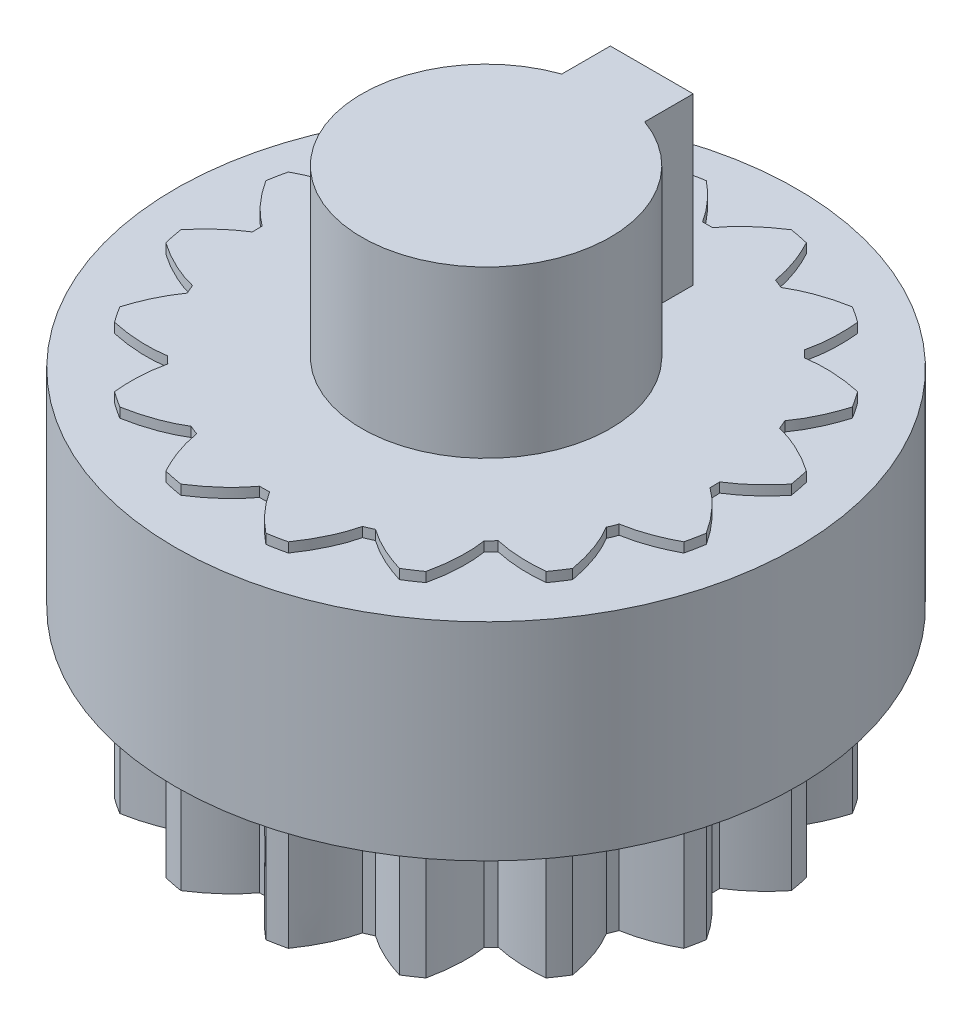
from build123d import *

# Parameters (mm, degrees)
BOSS_EXTRUDE1_DEPTH = 25
SKETCH2_R           = 15
BOSS_EXTRUDE2_DEPTH = 10
CUT_EXTRUDE1_START  = -8
CUT_EXTRUDE1_DEPTH  = 8


with BuildPart() as part:
    # Sketch1 → Boss-Extrude1 (new body)
    with BuildSketch(Plane(origin=(0, 0, 0), x_dir=(1, 0, 0), z_dir=(0, 1, 0))):
        with BuildLine():
            ThreePointArc((10.934408559, 6.749904405), (10.684384518, 7.139077494), (10.420515524, 7.518999682))
            add(Edge.make_bspline(
                [(7.734369608, 7.644942888), (7.815501047, 7.657706982), (8.159304568, 7.704570143), (8.788763458, 7.738663564), (9.465599617, 7.693246212), (10.052424346, 7.597679961), (10.374403818, 7.529145436), (10.420515524, 7.518999682)],
                knots=[0.024136697, 0.024136697, 0.024136697, 0.024136697, 0.024136697, 0.029959916, 0.048733667, 0.068727063, 0.072074856, 0.072074856, 0.072074856, 0.072074856, 0.072074856], degree=4))
            ThreePointArc((7.734369608, 7.644942888), (7.564424061, 7.813137246), (7.390821793, 7.977554652))
            add(Edge.make_bspline(
                [(7.390821793, 7.977554652), (7.395435654, 7.997349521), (7.458852977, 8.275301644), (7.549149712, 8.836196098), (7.580198449, 9.451763258), (7.554024219, 10.045742282), (7.523674581, 10.373532856), (7.518999682, 10.420515524)],
                knots=[0.028518712, 0.028518712, 0.028518712, 0.028518712, 0.028518712, 0.029959916, 0.048733667, 0.068727063, 0.072074856, 0.072074856, 0.072074856, 0.072074856, 0.072074856], degree=4))
            ThreePointArc((7.518999682, 10.420515524), (7.139077494, 10.684384518), (6.749904405, 10.934408559))
            add(Edge.make_bspline(
                [(4.220032793, 10.022821371), (4.290103862, 10.065661513), (4.589803143, 10.24052534), (5.15830034, 10.512907042), (5.800995883, 10.729960864), (6.37972286, 10.866237263), (6.703420131, 10.926135828), (6.749904405, 10.934408559)],
                knots=[0.024136697, 0.024136697, 0.024136697, 0.024136697, 0.024136697, 0.029959916, 0.048733667, 0.068727063, 0.072074856, 0.072074856, 0.072074856, 0.072074856, 0.072074856], degree=4))
            ThreePointArc((4.220032793, 10.022821371), (3.998658386, 10.11317735), (3.775350987, 10.198644514))
            add(Edge.make_bspline(
                [(3.775350987, 10.198644514), (3.77203847, 10.218698237), (3.724260764, 10.499761273), (3.593039055, 11.052515243), (3.386156994, 11.633106981), (3.134669227, 12.171855599), (2.981189795, 12.463080299), (2.958891263, 12.504697617)],
                knots=[0.028518712, 0.028518712, 0.028518712, 0.028518712, 0.028518712, 0.029959916, 0.048733667, 0.068727063, 0.072074856, 0.072074856, 0.072074856, 0.072074856, 0.072074856], degree=4))
            ThreePointArc((2.958891263, 12.504697617), (2.506910638, 12.603090853), (2.051681528, 12.685152853))
            add(Edge.make_bspline(
                [(0.06323424, 10.874816156), (0.111577253, 10.941210324), (0.321545796, 11.217453385), (0.742532756, 11.686655722), (1.253243112, 12.133136243), (1.735766401, 12.480508444), (2.011901496, 12.659721085), (2.051681528, 12.685152853)],
                knots=[0.024136697, 0.024136697, 0.024136697, 0.024136697, 0.024136697, 0.029959916, 0.048733667, 0.068727063, 0.072074856, 0.072074856, 0.072074856, 0.072074856, 0.072074856], degree=4))
            ThreePointArc((0.06323424, 10.874816156), (-0.17586678, 10.873577878), (-0.414882783, 10.8670832))
            add(Edge.make_bspline(
                [(-0.414882783, 10.8670832), (-0.425617377, 10.884342779), (-0.577316389, 11.125727429), (-0.910079227, 11.586189134), (-1.323396168, 12.04341562), (-1.761910739, 12.44491424), (-2.015154112, 12.655236743), (-2.051681528, 12.685152853)],
                knots=[0.028518712, 0.028518712, 0.028518712, 0.028518712, 0.028518712, 0.029959916, 0.048733667, 0.068727063, 0.072074856, 0.072074856, 0.072074856, 0.072074856, 0.072074856], degree=4))
            ThreePointArc((-2.051681528, 12.685152853), (-2.506910638, 12.603090853), (-2.958891263, 12.504697617))
            add(Edge.make_bspline(
                [(-4.103191153, 10.071218762), (-4.083935981, 10.151059045), (-3.995663984, 10.486625838), (-3.786278709, 11.081217009), (-3.485304562, 11.689151616), (-3.172444758, 12.194735351), (-2.985910904, 12.465978568), (-2.958891263, 12.504697617)],
                knots=[0.024136697, 0.024136697, 0.024136697, 0.024136697, 0.024136697, 0.029959916, 0.048733667, 0.068727063, 0.072074856, 0.072074856, 0.072074856, 0.072074856, 0.072074856], degree=4))
            ThreePointArc((-4.103191153, 10.071218762), (-4.323617823, 9.978574744), (-4.541954411, 9.881106979))
            add(Edge.make_bspline(
                [(-4.541954411, 9.881106979), (-4.558476837, 9.8929448), (-4.791002356, 10.057902438), (-5.274646197, 10.355970758), (-5.83147426, 10.620223405), (-6.390255767, 10.823347501), (-6.704709073, 10.920748114), (-6.749904405, 10.934408559)],
                knots=[0.028518712, 0.028518712, 0.028518712, 0.028518712, 0.028518712, 0.029959916, 0.048733667, 0.068727063, 0.072074856, 0.072074856, 0.072074856, 0.072074856, 0.072074856], degree=4))
            ThreePointArc((-6.749904405, 10.934408559), (-7.139077494, 10.684384518), (-7.518999682, 10.420515524))
            add(Edge.make_bspline(
                [(-7.644942888, 7.734369608), (-7.657706982, 7.815501047), (-7.704570143, 8.159304568), (-7.738663564, 8.788763458), (-7.693246212, 9.465599617), (-7.597679961, 10.052424346), (-7.529145436, 10.374403818), (-7.518999682, 10.420515524)],
                knots=[0.024136697, 0.024136697, 0.024136697, 0.024136697, 0.024136697, 0.029959916, 0.048733667, 0.068727063, 0.072074856, 0.072074856, 0.072074856, 0.072074856, 0.072074856], degree=4))
            ThreePointArc((-7.644942888, 7.734369608), (-7.813137246, 7.564424061), (-7.977554652, 7.390821793))
            add(Edge.make_bspline(
                [(-7.977554652, 7.390821793), (-7.997349521, 7.395435654), (-8.275301644, 7.458852977), (-8.836196098, 7.549149712), (-9.451763258, 7.580198449), (-10.045742282, 7.554024219), (-10.373532856, 7.523674581), (-10.420515524, 7.518999682)],
                knots=[0.028518712, 0.028518712, 0.028518712, 0.028518712, 0.028518712, 0.029959916, 0.048733667, 0.068727063, 0.072074856, 0.072074856, 0.072074856, 0.072074856, 0.072074856], degree=4))
            ThreePointArc((-10.420515524, 7.518999682), (-10.684384518, 7.139077494), (-10.934408559, 6.749904405))
            add(Edge.make_bspline(
                [(-10.022821371, 4.220032793), (-10.065661513, 4.290103862), (-10.24052534, 4.589803143), (-10.512907042, 5.15830034), (-10.729960864, 5.800995883), (-10.866237263, 6.37972286), (-10.926135828, 6.703420131), (-10.934408559, 6.749904405)],
                knots=[0.024136697, 0.024136697, 0.024136697, 0.024136697, 0.024136697, 0.029959916, 0.048733667, 0.068727063, 0.072074856, 0.072074856, 0.072074856, 0.072074856, 0.072074856], degree=4))
            ThreePointArc((-10.022821371, 4.220032793), (-10.11317735, 3.998658386), (-10.198644514, 3.775350987))
            add(Edge.make_bspline(
                [(-10.198644514, 3.775350987), (-10.218698237, 3.77203847), (-10.499761273, 3.724260764), (-11.052515243, 3.593039055), (-11.633106981, 3.386156994), (-12.171855599, 3.134669227), (-12.463080299, 2.981189795), (-12.504697617, 2.958891263)],
                knots=[0.028518712, 0.028518712, 0.028518712, 0.028518712, 0.028518712, 0.029959916, 0.048733667, 0.068727063, 0.072074856, 0.072074856, 0.072074856, 0.072074856, 0.072074856], degree=4))
            ThreePointArc((-12.504697617, 2.958891263), (-12.603090853, 2.506910638), (-12.685152853, 2.051681528))
            add(Edge.make_bspline(
                [(-10.874816156, 0.06323424), (-10.941210324, 0.111577253), (-11.217453385, 0.321545796), (-11.686655722, 0.742532756), (-12.133136243, 1.253243112), (-12.480508444, 1.735766401), (-12.659721085, 2.011901496), (-12.685152853, 2.051681528)],
                knots=[0.024136697, 0.024136697, 0.024136697, 0.024136697, 0.024136697, 0.029959916, 0.048733667, 0.068727063, 0.072074856, 0.072074856, 0.072074856, 0.072074856, 0.072074856], degree=4))
            ThreePointArc((-10.874816156, 0.06323424), (-10.873577878, -0.17586678), (-10.8670832, -0.414882783))
            add(Edge.make_bspline(
                [(-10.8670832, -0.414882783), (-10.884342779, -0.425617377), (-11.125727429, -0.577316389), (-11.586189134, -0.910079227), (-12.04341562, -1.323396168), (-12.44491424, -1.761910739), (-12.655236743, -2.015154112), (-12.685152853, -2.051681528)],
                knots=[0.028518712, 0.028518712, 0.028518712, 0.028518712, 0.028518712, 0.029959916, 0.048733667, 0.068727063, 0.072074856, 0.072074856, 0.072074856, 0.072074856, 0.072074856], degree=4))
            ThreePointArc((-12.685152853, -2.051681528), (-12.603090853, -2.506910638), (-12.504697617, -2.958891263))
            add(Edge.make_bspline(
                [(-10.071218762, -4.103191153), (-10.151059045, -4.083935981), (-10.486625838, -3.995663984), (-11.081217009, -3.786278709), (-11.689151616, -3.485304562), (-12.194735351, -3.172444758), (-12.465978568, -2.985910904), (-12.504697617, -2.958891263)],
                knots=[0.024136697, 0.024136697, 0.024136697, 0.024136697, 0.024136697, 0.029959916, 0.048733667, 0.068727063, 0.072074856, 0.072074856, 0.072074856, 0.072074856, 0.072074856], degree=4))
            ThreePointArc((-10.071218762, -4.103191153), (-9.978574744, -4.323617823), (-9.881106979, -4.541954411))
            add(Edge.make_bspline(
                [(-9.881106979, -4.541954411), (-9.8929448, -4.558476837), (-10.057902438, -4.791002356), (-10.355970758, -5.274646197), (-10.620223405, -5.83147426), (-10.823347501, -6.390255767), (-10.920748114, -6.704709073), (-10.934408559, -6.749904405)],
                knots=[0.028518712, 0.028518712, 0.028518712, 0.028518712, 0.028518712, 0.029959916, 0.048733667, 0.068727063, 0.072074856, 0.072074856, 0.072074856, 0.072074856, 0.072074856], degree=4))
            ThreePointArc((-10.934408559, -6.749904405), (-10.684384518, -7.139077494), (-10.420515524, -7.518999682))
            add(Edge.make_bspline(
                [(-7.734369608, -7.644942888), (-7.815501047, -7.657706982), (-8.159304568, -7.704570143), (-8.788763458, -7.738663564), (-9.465599617, -7.693246212), (-10.052424346, -7.597679961), (-10.374403818, -7.529145436), (-10.420515524, -7.518999682)],
                knots=[0.024136697, 0.024136697, 0.024136697, 0.024136697, 0.024136697, 0.029959916, 0.048733667, 0.068727063, 0.072074856, 0.072074856, 0.072074856, 0.072074856, 0.072074856], degree=4))
            ThreePointArc((-7.734369608, -7.644942888), (-7.564424061, -7.813137246), (-7.390821793, -7.977554652))
            add(Edge.make_bspline(
                [(-7.390821793, -7.977554652), (-7.395435654, -7.997349521), (-7.458852977, -8.275301644), (-7.549149712, -8.836196098), (-7.580198449, -9.451763258), (-7.554024219, -10.045742282), (-7.523674581, -10.373532856), (-7.518999682, -10.420515524)],
                knots=[0.028518712, 0.028518712, 0.028518712, 0.028518712, 0.028518712, 0.029959916, 0.048733667, 0.068727063, 0.072074856, 0.072074856, 0.072074856, 0.072074856, 0.072074856], degree=4))
            ThreePointArc((-7.518999682, -10.420515524), (-7.139077494, -10.684384518), (-6.749904405, -10.934408559))
            add(Edge.make_bspline(
                [(-4.220032793, -10.022821371), (-4.290103862, -10.065661513), (-4.589803143, -10.24052534), (-5.15830034, -10.512907042), (-5.800995883, -10.729960864), (-6.37972286, -10.866237263), (-6.703420131, -10.926135828), (-6.749904405, -10.934408559)],
                knots=[0.024136697, 0.024136697, 0.024136697, 0.024136697, 0.024136697, 0.029959916, 0.048733667, 0.068727063, 0.072074856, 0.072074856, 0.072074856, 0.072074856, 0.072074856], degree=4))
            ThreePointArc((-4.220032793, -10.022821371), (-3.998658386, -10.11317735), (-3.775350987, -10.198644514))
            add(Edge.make_bspline(
                [(-3.775350987, -10.198644514), (-3.77203847, -10.218698237), (-3.724260764, -10.499761273), (-3.593039055, -11.052515243), (-3.386156994, -11.633106981), (-3.134669227, -12.171855599), (-2.981189795, -12.463080299), (-2.958891263, -12.504697617)],
                knots=[0.028518712, 0.028518712, 0.028518712, 0.028518712, 0.028518712, 0.029959916, 0.048733667, 0.068727063, 0.072074856, 0.072074856, 0.072074856, 0.072074856, 0.072074856], degree=4))
            ThreePointArc((-2.958891263, -12.504697617), (-2.506910638, -12.603090853), (-2.051681528, -12.685152853))
            add(Edge.make_bspline(
                [(-0.06323424, -10.874816156), (-0.111577253, -10.941210324), (-0.321545796, -11.217453385), (-0.742532756, -11.686655722), (-1.253243112, -12.133136243), (-1.735766401, -12.480508444), (-2.011901496, -12.659721085), (-2.051681528, -12.685152853)],
                knots=[0.024136697, 0.024136697, 0.024136697, 0.024136697, 0.024136697, 0.029959916, 0.048733667, 0.068727063, 0.072074856, 0.072074856, 0.072074856, 0.072074856, 0.072074856], degree=4))
            ThreePointArc((-0.06323424, -10.874816156), (0.17586678, -10.873577878), (0.414882783, -10.8670832))
            add(Edge.make_bspline(
                [(0.414882783, -10.8670832), (0.425617377, -10.884342779), (0.577316389, -11.125727429), (0.910079227, -11.586189134), (1.323396168, -12.04341562), (1.761910739, -12.44491424), (2.015154112, -12.655236743), (2.051681528, -12.685152853)],
                knots=[0.028518712, 0.028518712, 0.028518712, 0.028518712, 0.028518712, 0.029959916, 0.048733667, 0.068727063, 0.072074856, 0.072074856, 0.072074856, 0.072074856, 0.072074856], degree=4))
            ThreePointArc((2.051681528, -12.685152853), (2.506910638, -12.603090853), (2.958891263, -12.504697617))
            add(Edge.make_bspline(
                [(4.103191153, -10.071218762), (4.083935981, -10.151059045), (3.995663984, -10.486625838), (3.786278709, -11.081217009), (3.485304562, -11.689151616), (3.172444758, -12.194735351), (2.985910904, -12.465978568), (2.958891263, -12.504697617)],
                knots=[0.024136697, 0.024136697, 0.024136697, 0.024136697, 0.024136697, 0.029959916, 0.048733667, 0.068727063, 0.072074856, 0.072074856, 0.072074856, 0.072074856, 0.072074856], degree=4))
            ThreePointArc((4.103191153, -10.071218762), (4.323617823, -9.978574744), (4.541954411, -9.881106979))
            add(Edge.make_bspline(
                [(4.541954411, -9.881106979), (4.558476837, -9.8929448), (4.791002356, -10.057902438), (5.274646197, -10.355970758), (5.83147426, -10.620223405), (6.390255767, -10.823347501), (6.704709073, -10.920748114), (6.749904405, -10.934408559)],
                knots=[0.028518712, 0.028518712, 0.028518712, 0.028518712, 0.028518712, 0.029959916, 0.048733667, 0.068727063, 0.072074856, 0.072074856, 0.072074856, 0.072074856, 0.072074856], degree=4))
            ThreePointArc((6.749904405, -10.934408559), (7.139077494, -10.684384518), (7.518999682, -10.420515524))
            add(Edge.make_bspline(
                [(7.644942888, -7.734369608), (7.657706982, -7.815501047), (7.704570143, -8.159304568), (7.738663564, -8.788763458), (7.693246212, -9.465599617), (7.597679961, -10.052424346), (7.529145436, -10.374403818), (7.518999682, -10.420515524)],
                knots=[0.024136697, 0.024136697, 0.024136697, 0.024136697, 0.024136697, 0.029959916, 0.048733667, 0.068727063, 0.072074856, 0.072074856, 0.072074856, 0.072074856, 0.072074856], degree=4))
            ThreePointArc((7.644942888, -7.734369608), (7.813137246, -7.564424061), (7.977554652, -7.390821793))
            add(Edge.make_bspline(
                [(7.977554652, -7.390821793), (7.997349521, -7.395435654), (8.275301644, -7.458852977), (8.836196098, -7.549149712), (9.451763258, -7.580198449), (10.045742282, -7.554024219), (10.373532856, -7.523674581), (10.420515524, -7.518999682)],
                knots=[0.028518712, 0.028518712, 0.028518712, 0.028518712, 0.028518712, 0.029959916, 0.048733667, 0.068727063, 0.072074856, 0.072074856, 0.072074856, 0.072074856, 0.072074856], degree=4))
            ThreePointArc((10.420515524, -7.518999682), (10.684384518, -7.139077494), (10.934408559, -6.749904405))
            add(Edge.make_bspline(
                [(10.022821371, -4.220032793), (10.065661513, -4.290103862), (10.24052534, -4.589803143), (10.512907042, -5.15830034), (10.729960864, -5.800995883), (10.866237263, -6.37972286), (10.926135828, -6.703420131), (10.934408559, -6.749904405)],
                knots=[0.024136697, 0.024136697, 0.024136697, 0.024136697, 0.024136697, 0.029959916, 0.048733667, 0.068727063, 0.072074856, 0.072074856, 0.072074856, 0.072074856, 0.072074856], degree=4))
            ThreePointArc((10.022821371, -4.220032793), (10.11317735, -3.998658386), (10.198644514, -3.775350987))
            add(Edge.make_bspline(
                [(10.198644514, -3.775350987), (10.218698237, -3.77203847), (10.499761273, -3.724260764), (11.052515243, -3.593039055), (11.633106981, -3.386156994), (12.171855599, -3.134669227), (12.463080299, -2.981189795), (12.504697617, -2.958891263)],
                knots=[0.028518712, 0.028518712, 0.028518712, 0.028518712, 0.028518712, 0.029959916, 0.048733667, 0.068727063, 0.072074856, 0.072074856, 0.072074856, 0.072074856, 0.072074856], degree=4))
            ThreePointArc((12.504697617, -2.958891263), (12.603090853, -2.506910638), (12.685152853, -2.051681528))
            add(Edge.make_bspline(
                [(10.874816156, -0.06323424), (10.941210324, -0.111577253), (11.217453385, -0.321545796), (11.686655722, -0.742532756), (12.133136243, -1.253243112), (12.480508444, -1.735766401), (12.659721085, -2.011901496), (12.685152853, -2.051681528)],
                knots=[0.024136697, 0.024136697, 0.024136697, 0.024136697, 0.024136697, 0.029959916, 0.048733667, 0.068727063, 0.072074856, 0.072074856, 0.072074856, 0.072074856, 0.072074856], degree=4))
            ThreePointArc((10.874816156, -0.06323424), (10.8735779, 0.175865412), (10.867083304, 0.41488005))
            add(Edge.make_bspline(
                [(10.867083304, 0.41488005), (10.881563831, 0.423886532), (10.909967193, 0.441770581), (10.976624087, 0.484202292), (11.030614279, 0.520337558), (11.104594394, 0.570140428), (11.165588686, 0.613063664), (11.233528062, 0.661496019), (11.296306007, 0.707854009), (11.361321254, 0.756764897), (11.424005499, 0.805285781), (11.487262257, 0.855332478), (11.549125239, 0.905448576), (11.611116576, 0.956904432), (11.682171109, 1.017033988), (11.768675064, 1.092619353), (11.8667636, 1.180577496), (11.981028216, 1.288212398), (12.092602454, 1.396325305), (12.209848472, 1.516302043), (12.31227485, 1.623029301), (12.43305143, 1.756891779), (12.517769899, 1.851362852), (12.621696804, 1.974933325), (12.663559289, 2.025313794), (12.685153092, 2.05168005)],
                knots=[0.063770479, 0.063770479, 0.063770479, 0.063770479, 0.063770479, 0.091530707, 0.119271063, 0.147011529, 0.174751886, 0.202492214, 0.230232656, 0.257973071, 0.285713397, 0.313453819, 0.341194243, 0.368934578, 0.396674935, 0.424415392, 0.47104384, 0.526524589, 0.58200537, 0.637486135, 0.692966903, 0.748447704, 0.803928446, 0.859409239, 0.914890039, 0.914890039, 0.914890039, 0.914890039, 0.914890039], degree=4))
            ThreePointArc((12.685153092, 2.05168005), (12.603090999, 2.506909904), (12.504697617, 2.958891263))
            add(Edge.make_bspline(
                [(10.071218762, 4.103191153), (10.151059045, 4.083935981), (10.486625838, 3.995663984), (11.081217009, 3.786278709), (11.689151616, 3.485304562), (12.194735351, 3.172444758), (12.465978568, 2.985910904), (12.504697617, 2.958891263)],
                knots=[0.024136697, 0.024136697, 0.024136697, 0.024136697, 0.024136697, 0.029959916, 0.048733667, 0.068727063, 0.072074856, 0.072074856, 0.072074856, 0.072074856, 0.072074856], degree=4))
            ThreePointArc((10.071218762, 4.103191153), (9.978574744, 4.323617823), (9.881106979, 4.541954411))
            add(Edge.make_bspline(
                [(9.881106979, 4.541954411), (9.8929448, 4.558476837), (10.057902438, 4.791002356), (10.355970758, 5.274646197), (10.620223405, 5.83147426), (10.823347501, 6.390255767), (10.920748114, 6.704709073), (10.934408559, 6.749904405)],
                knots=[0.028518712, 0.028518712, 0.028518712, 0.028518712, 0.028518712, 0.029959916, 0.048733667, 0.068727063, 0.072074856, 0.072074856, 0.072074856, 0.072074856, 0.072074856], degree=4))
        make_face()
    extrude(amount=BOSS_EXTRUDE1_DEPTH)

    # Sketch2 → Boss-Extrude2 (add)
    with BuildSketch(Plane(origin=(0, 6.530075329, 0), x_dir=(1, 0, 0), z_dir=(0, 1, 0))):
        with Locations(Location((0, 0, 0), (0, 0, 270))):
            Circle(SKETCH2_R)
    extrude(amount=BOSS_EXTRUDE2_DEPTH)

    # Sketch3 → Cut-Extrude1 (cut)
    with BuildSketch(Plane(origin=(0, 25, 0), x_dir=(1, 0, 0), z_dir=(0, 1, 0)).offset(CUT_EXTRUDE1_START)):
        with BuildLine():
            ThreePointArc((10.874816156, -0.06323424), (10.8735779, 0.175865412), (10.867083304, 0.41488005))
            add(Edge.make_bspline(
                [(10.867083304, 0.41488005), (10.881563831, 0.423886532), (10.909967193, 0.441770581), (10.976624087, 0.484202292), (11.030614279, 0.520337558), (11.104594394, 0.570140428), (11.165588686, 0.613063664), (11.233528062, 0.661496019), (11.296306007, 0.707854009), (11.361321254, 0.756764897), (11.424005499, 0.805285781), (11.487262257, 0.855332478), (11.549125239, 0.905448576), (11.611116576, 0.956904432), (11.682171109, 1.017033988), (11.768675064, 1.092619353), (11.8667636, 1.180577496), (11.981028216, 1.288212398), (12.092602454, 1.396325305), (12.209848472, 1.516302043), (12.31227485, 1.623029301), (12.43305143, 1.756891779), (12.517769899, 1.851362852), (12.621696804, 1.974933325), (12.663559289, 2.025313794), (12.685153092, 2.05168005)],
                knots=[0.063770479, 0.063770479, 0.063770479, 0.063770479, 0.063770479, 0.091530707, 0.119271063, 0.147011529, 0.174751886, 0.202492214, 0.230232656, 0.257973071, 0.285713397, 0.313453819, 0.341194243, 0.368934578, 0.396674935, 0.424415392, 0.47104384, 0.526524589, 0.58200537, 0.637486135, 0.692966903, 0.748447704, 0.803928446, 0.859409239, 0.914890039, 0.914890039, 0.914890039, 0.914890039, 0.914890039], degree=4))
            ThreePointArc((12.685153092, 2.05168005), (12.603090999, 2.506909904), (12.504697617, 2.958891263))
            add(Edge.make_bspline(
                [(12.504697617, 2.958891263), (12.465978568, 2.985910904), (12.194735351, 3.172444758), (11.689151616, 3.485304562), (11.081217009, 3.786278709), (10.486625838, 3.995663984), (10.151059045, 4.083935981), (10.071218762, 4.103191153)],
                knots=[0.024136697, 0.024136697, 0.024136697, 0.024136697, 0.024136697, 0.02748449, 0.047477886, 0.066251637, 0.072074856, 0.072074856, 0.072074856, 0.072074856, 0.072074856], degree=4))
            ThreePointArc((10.071218762, 4.103191153), (9.978574744, 4.323617823), (9.881106979, 4.541954411))
            add(Edge.make_bspline(
                [(9.881106979, 4.541954411), (9.8929448, 4.558476837), (10.057902438, 4.791002356), (10.355970758, 5.274646197), (10.620223405, 5.83147426), (10.823347501, 6.390255767), (10.920748114, 6.704709073), (10.934408559, 6.749904405)],
                knots=[0.028518712, 0.028518712, 0.028518712, 0.028518712, 0.028518712, 0.029959916, 0.048733667, 0.068727063, 0.072074856, 0.072074856, 0.072074856, 0.072074856, 0.072074856], degree=4))
            ThreePointArc((10.934408559, 6.749904405), (10.684384518, 7.139077494), (10.420515524, 7.518999682))
            add(Edge.make_bspline(
                [(10.420515524, 7.518999682), (10.374403818, 7.529145436), (10.052424346, 7.597679961), (9.465599617, 7.693246212), (8.788763458, 7.738663564), (8.159304568, 7.704570143), (7.815501047, 7.657706982), (7.734369608, 7.644942888)],
                knots=[0.024136697, 0.024136697, 0.024136697, 0.024136697, 0.024136697, 0.02748449, 0.047477886, 0.066251637, 0.072074856, 0.072074856, 0.072074856, 0.072074856, 0.072074856], degree=4))
            ThreePointArc((7.734369608, 7.644942888), (7.564424061, 7.813137246), (7.390821793, 7.977554652))
            add(Edge.make_bspline(
                [(7.390821793, 7.977554652), (7.395435654, 7.997349521), (7.458852977, 8.275301644), (7.549149712, 8.836196098), (7.580198449, 9.451763258), (7.554024219, 10.045742282), (7.523674581, 10.373532856), (7.518999682, 10.420515524)],
                knots=[0.028518712, 0.028518712, 0.028518712, 0.028518712, 0.028518712, 0.029959916, 0.048733667, 0.068727063, 0.072074856, 0.072074856, 0.072074856, 0.072074856, 0.072074856], degree=4))
            ThreePointArc((7.518999682, 10.420515524), (7.139077494, 10.684384518), (6.749904405, 10.934408559))
            add(Edge.make_bspline(
                [(6.749904405, 10.934408559), (6.703420131, 10.926135828), (6.37972286, 10.866237263), (5.800995883, 10.729960864), (5.15830034, 10.512907042), (4.589803143, 10.24052534), (4.290103862, 10.065661513), (4.220032793, 10.022821371)],
                knots=[0.024136697, 0.024136697, 0.024136697, 0.024136697, 0.024136697, 0.02748449, 0.047477886, 0.066251637, 0.072074856, 0.072074856, 0.072074856, 0.072074856, 0.072074856], degree=4))
            ThreePointArc((4.220032793, 10.022821371), (3.998658386, 10.11317735), (3.775350987, 10.198644514))
            add(Edge.make_bspline(
                [(3.775350987, 10.198644514), (3.77203847, 10.218698237), (3.724260764, 10.499761273), (3.593039055, 11.052515243), (3.386156994, 11.633106981), (3.134669227, 12.171855599), (2.981189795, 12.463080299), (2.958891263, 12.504697617)],
                knots=[0.028518712, 0.028518712, 0.028518712, 0.028518712, 0.028518712, 0.029959916, 0.048733667, 0.068727063, 0.072074856, 0.072074856, 0.072074856, 0.072074856, 0.072074856], degree=4))
            ThreePointArc((2.958891263, 12.504697617), (2.506910638, 12.603090853), (2.051681528, 12.685152853))
            add(Edge.make_bspline(
                [(2.051681528, 12.685152853), (2.011901496, 12.659721085), (1.735766401, 12.480508444), (1.253243112, 12.133136243), (0.742532756, 11.686655722), (0.321545796, 11.217453385), (0.111577253, 10.941210324), (0.06323424, 10.874816156)],
                knots=[0.024136697, 0.024136697, 0.024136697, 0.024136697, 0.024136697, 0.02748449, 0.047477886, 0.066251637, 0.072074856, 0.072074856, 0.072074856, 0.072074856, 0.072074856], degree=4))
            ThreePointArc((0.06323424, 10.874816156), (-0.17586678, 10.873577878), (-0.414882783, 10.8670832))
            add(Edge.make_bspline(
                [(-0.414882783, 10.8670832), (-0.425617377, 10.884342779), (-0.577316389, 11.125727429), (-0.910079227, 11.586189134), (-1.323396168, 12.04341562), (-1.761910739, 12.44491424), (-2.015154112, 12.655236743), (-2.051681528, 12.685152853)],
                knots=[0.028518712, 0.028518712, 0.028518712, 0.028518712, 0.028518712, 0.029959916, 0.048733667, 0.068727063, 0.072074856, 0.072074856, 0.072074856, 0.072074856, 0.072074856], degree=4))
            ThreePointArc((-2.051681528, 12.685152853), (-2.506910638, 12.603090853), (-2.958891263, 12.504697617))
            add(Edge.make_bspline(
                [(-2.958891263, 12.504697617), (-2.985910904, 12.465978568), (-3.172444758, 12.194735351), (-3.485304562, 11.689151616), (-3.786278709, 11.081217009), (-3.995663984, 10.486625838), (-4.083935981, 10.151059045), (-4.103191153, 10.071218762)],
                knots=[0.024136697, 0.024136697, 0.024136697, 0.024136697, 0.024136697, 0.02748449, 0.047477886, 0.066251637, 0.072074856, 0.072074856, 0.072074856, 0.072074856, 0.072074856], degree=4))
            ThreePointArc((-4.103191153, 10.071218762), (-4.323617823, 9.978574744), (-4.541954411, 9.881106979))
            add(Edge.make_bspline(
                [(-4.541954411, 9.881106979), (-4.558476837, 9.8929448), (-4.791002356, 10.057902438), (-5.274646197, 10.355970758), (-5.83147426, 10.620223405), (-6.390255767, 10.823347501), (-6.704709073, 10.920748114), (-6.749904405, 10.934408559)],
                knots=[0.028518712, 0.028518712, 0.028518712, 0.028518712, 0.028518712, 0.029959916, 0.048733667, 0.068727063, 0.072074856, 0.072074856, 0.072074856, 0.072074856, 0.072074856], degree=4))
            ThreePointArc((-6.749904405, 10.934408559), (-7.139077494, 10.684384518), (-7.518999682, 10.420515524))
            add(Edge.make_bspline(
                [(-7.518999682, 10.420515524), (-7.529145436, 10.374403818), (-7.597679961, 10.052424346), (-7.693246212, 9.465599617), (-7.738663564, 8.788763458), (-7.704570143, 8.159304568), (-7.657706982, 7.815501047), (-7.644942888, 7.734369608)],
                knots=[0.024136697, 0.024136697, 0.024136697, 0.024136697, 0.024136697, 0.02748449, 0.047477886, 0.066251637, 0.072074856, 0.072074856, 0.072074856, 0.072074856, 0.072074856], degree=4))
            ThreePointArc((-7.644942888, 7.734369608), (-7.813137246, 7.564424061), (-7.977554652, 7.390821793))
            add(Edge.make_bspline(
                [(-7.977554652, 7.390821793), (-7.997349521, 7.395435654), (-8.275301644, 7.458852977), (-8.836196098, 7.549149712), (-9.451763258, 7.580198449), (-10.045742282, 7.554024219), (-10.373532856, 7.523674581), (-10.420515524, 7.518999682)],
                knots=[0.028518712, 0.028518712, 0.028518712, 0.028518712, 0.028518712, 0.029959916, 0.048733667, 0.068727063, 0.072074856, 0.072074856, 0.072074856, 0.072074856, 0.072074856], degree=4))
            ThreePointArc((-10.420515524, 7.518999682), (-10.684384518, 7.139077494), (-10.934408559, 6.749904405))
            add(Edge.make_bspline(
                [(-10.934408559, 6.749904405), (-10.926135828, 6.703420131), (-10.866237263, 6.37972286), (-10.729960864, 5.800995883), (-10.512907042, 5.15830034), (-10.24052534, 4.589803143), (-10.065661513, 4.290103862), (-10.022821371, 4.220032793)],
                knots=[0.024136697, 0.024136697, 0.024136697, 0.024136697, 0.024136697, 0.02748449, 0.047477886, 0.066251637, 0.072074856, 0.072074856, 0.072074856, 0.072074856, 0.072074856], degree=4))
            ThreePointArc((-10.022821371, 4.220032793), (-10.11317735, 3.998658386), (-10.198644514, 3.775350987))
            add(Edge.make_bspline(
                [(-10.198644514, 3.775350987), (-10.218698237, 3.77203847), (-10.499761273, 3.724260764), (-11.052515243, 3.593039055), (-11.633106981, 3.386156994), (-12.171855599, 3.134669227), (-12.463080299, 2.981189795), (-12.504697617, 2.958891263)],
                knots=[0.028518712, 0.028518712, 0.028518712, 0.028518712, 0.028518712, 0.029959916, 0.048733667, 0.068727063, 0.072074856, 0.072074856, 0.072074856, 0.072074856, 0.072074856], degree=4))
            ThreePointArc((-12.504697617, 2.958891263), (-12.603090853, 2.506910638), (-12.685152853, 2.051681528))
            add(Edge.make_bspline(
                [(-12.685152853, 2.051681528), (-12.659721085, 2.011901496), (-12.480508444, 1.735766401), (-12.133136243, 1.253243112), (-11.686655722, 0.742532756), (-11.217453385, 0.321545796), (-10.941210324, 0.111577253), (-10.874816156, 0.06323424)],
                knots=[0.024136697, 0.024136697, 0.024136697, 0.024136697, 0.024136697, 0.02748449, 0.047477886, 0.066251637, 0.072074856, 0.072074856, 0.072074856, 0.072074856, 0.072074856], degree=4))
            ThreePointArc((-10.874816156, 0.06323424), (-10.873577878, -0.17586678), (-10.8670832, -0.414882783))
            add(Edge.make_bspline(
                [(-10.8670832, -0.414882783), (-10.884342779, -0.425617377), (-11.125727429, -0.577316389), (-11.586189134, -0.910079227), (-12.04341562, -1.323396168), (-12.44491424, -1.761910739), (-12.655236743, -2.015154112), (-12.685152853, -2.051681528)],
                knots=[0.028518712, 0.028518712, 0.028518712, 0.028518712, 0.028518712, 0.029959916, 0.048733667, 0.068727063, 0.072074856, 0.072074856, 0.072074856, 0.072074856, 0.072074856], degree=4))
            ThreePointArc((-12.685152853, -2.051681528), (-12.603090853, -2.506910638), (-12.504697617, -2.958891263))
            add(Edge.make_bspline(
                [(-12.504697617, -2.958891263), (-12.465978568, -2.985910904), (-12.194735351, -3.172444758), (-11.689151616, -3.485304562), (-11.081217009, -3.786278709), (-10.486625838, -3.995663984), (-10.151059045, -4.083935981), (-10.071218762, -4.103191153)],
                knots=[0.024136697, 0.024136697, 0.024136697, 0.024136697, 0.024136697, 0.02748449, 0.047477886, 0.066251637, 0.072074856, 0.072074856, 0.072074856, 0.072074856, 0.072074856], degree=4))
            ThreePointArc((-10.071218762, -4.103191153), (-9.978574744, -4.323617823), (-9.881106979, -4.541954411))
            add(Edge.make_bspline(
                [(-9.881106979, -4.541954411), (-9.8929448, -4.558476837), (-10.057902438, -4.791002356), (-10.355970758, -5.274646197), (-10.620223405, -5.83147426), (-10.823347501, -6.390255767), (-10.920748114, -6.704709073), (-10.934408559, -6.749904405)],
                knots=[0.028518712, 0.028518712, 0.028518712, 0.028518712, 0.028518712, 0.029959916, 0.048733667, 0.068727063, 0.072074856, 0.072074856, 0.072074856, 0.072074856, 0.072074856], degree=4))
            ThreePointArc((-10.934408559, -6.749904405), (-10.684384518, -7.139077494), (-10.420515524, -7.518999682))
            add(Edge.make_bspline(
                [(-10.420515524, -7.518999682), (-10.374403818, -7.529145436), (-10.052424346, -7.597679961), (-9.465599617, -7.693246212), (-8.788763458, -7.738663564), (-8.159304568, -7.704570143), (-7.815501047, -7.657706982), (-7.734369608, -7.644942888)],
                knots=[0.024136697, 0.024136697, 0.024136697, 0.024136697, 0.024136697, 0.02748449, 0.047477886, 0.066251637, 0.072074856, 0.072074856, 0.072074856, 0.072074856, 0.072074856], degree=4))
            ThreePointArc((-7.734369608, -7.644942888), (-7.564424061, -7.813137246), (-7.390821793, -7.977554652))
            add(Edge.make_bspline(
                [(-7.390821793, -7.977554652), (-7.395435654, -7.997349521), (-7.458852977, -8.275301644), (-7.549149712, -8.836196098), (-7.580198449, -9.451763258), (-7.554024219, -10.045742282), (-7.523674581, -10.373532856), (-7.518999682, -10.420515524)],
                knots=[0.028518712, 0.028518712, 0.028518712, 0.028518712, 0.028518712, 0.029959916, 0.048733667, 0.068727063, 0.072074856, 0.072074856, 0.072074856, 0.072074856, 0.072074856], degree=4))
            ThreePointArc((-7.518999682, -10.420515524), (-7.139077494, -10.684384518), (-6.749904405, -10.934408559))
            add(Edge.make_bspline(
                [(-6.749904405, -10.934408559), (-6.703420131, -10.926135828), (-6.37972286, -10.866237263), (-5.800995883, -10.729960864), (-5.15830034, -10.512907042), (-4.589803143, -10.24052534), (-4.290103862, -10.065661513), (-4.220032793, -10.022821371)],
                knots=[0.024136697, 0.024136697, 0.024136697, 0.024136697, 0.024136697, 0.02748449, 0.047477886, 0.066251637, 0.072074856, 0.072074856, 0.072074856, 0.072074856, 0.072074856], degree=4))
            ThreePointArc((-4.220032793, -10.022821371), (-3.998658386, -10.11317735), (-3.775350987, -10.198644514))
            add(Edge.make_bspline(
                [(-3.775350987, -10.198644514), (-3.77203847, -10.218698237), (-3.724260764, -10.499761273), (-3.593039055, -11.052515243), (-3.386156994, -11.633106981), (-3.134669227, -12.171855599), (-2.981189795, -12.463080299), (-2.958891263, -12.504697617)],
                knots=[0.028518712, 0.028518712, 0.028518712, 0.028518712, 0.028518712, 0.029959916, 0.048733667, 0.068727063, 0.072074856, 0.072074856, 0.072074856, 0.072074856, 0.072074856], degree=4))
            ThreePointArc((-2.958891263, -12.504697617), (-2.506910638, -12.603090853), (-2.051681528, -12.685152853))
            add(Edge.make_bspline(
                [(-2.051681528, -12.685152853), (-2.011901496, -12.659721085), (-1.735766401, -12.480508444), (-1.253243112, -12.133136243), (-0.742532756, -11.686655722), (-0.321545796, -11.217453385), (-0.111577253, -10.941210324), (-0.06323424, -10.874816156)],
                knots=[0.024136697, 0.024136697, 0.024136697, 0.024136697, 0.024136697, 0.02748449, 0.047477886, 0.066251637, 0.072074856, 0.072074856, 0.072074856, 0.072074856, 0.072074856], degree=4))
            ThreePointArc((-0.06323424, -10.874816156), (0.17586678, -10.873577878), (0.414882783, -10.8670832))
            add(Edge.make_bspline(
                [(0.414882783, -10.8670832), (0.425617377, -10.884342779), (0.577316389, -11.125727429), (0.910079227, -11.586189134), (1.323396168, -12.04341562), (1.761910739, -12.44491424), (2.015154112, -12.655236743), (2.051681528, -12.685152853)],
                knots=[0.028518712, 0.028518712, 0.028518712, 0.028518712, 0.028518712, 0.029959916, 0.048733667, 0.068727063, 0.072074856, 0.072074856, 0.072074856, 0.072074856, 0.072074856], degree=4))
            ThreePointArc((2.051681528, -12.685152853), (2.506910638, -12.603090853), (2.958891263, -12.504697617))
            add(Edge.make_bspline(
                [(2.958891263, -12.504697617), (2.985910904, -12.465978568), (3.172444758, -12.194735351), (3.485304562, -11.689151616), (3.786278709, -11.081217009), (3.995663984, -10.486625838), (4.083935981, -10.151059045), (4.103191153, -10.071218762)],
                knots=[0.024136697, 0.024136697, 0.024136697, 0.024136697, 0.024136697, 0.02748449, 0.047477886, 0.066251637, 0.072074856, 0.072074856, 0.072074856, 0.072074856, 0.072074856], degree=4))
            ThreePointArc((4.103191153, -10.071218762), (4.323617823, -9.978574744), (4.541954411, -9.881106979))
            add(Edge.make_bspline(
                [(4.541954411, -9.881106979), (4.558476837, -9.8929448), (4.791002356, -10.057902438), (5.274646197, -10.355970758), (5.83147426, -10.620223405), (6.390255767, -10.823347501), (6.704709073, -10.920748114), (6.749904405, -10.934408559)],
                knots=[0.028518712, 0.028518712, 0.028518712, 0.028518712, 0.028518712, 0.029959916, 0.048733667, 0.068727063, 0.072074856, 0.072074856, 0.072074856, 0.072074856, 0.072074856], degree=4))
            ThreePointArc((6.749904405, -10.934408559), (7.139077494, -10.684384518), (7.518999682, -10.420515524))
            add(Edge.make_bspline(
                [(7.518999682, -10.420515524), (7.529145436, -10.374403818), (7.597679961, -10.052424346), (7.693246212, -9.465599617), (7.738663564, -8.788763458), (7.704570143, -8.159304568), (7.657706982, -7.815501047), (7.644942888, -7.734369608)],
                knots=[0.024136697, 0.024136697, 0.024136697, 0.024136697, 0.024136697, 0.02748449, 0.047477886, 0.066251637, 0.072074856, 0.072074856, 0.072074856, 0.072074856, 0.072074856], degree=4))
            ThreePointArc((7.644942888, -7.734369608), (7.813137246, -7.564424061), (7.977554652, -7.390821793))
            add(Edge.make_bspline(
                [(7.977554652, -7.390821793), (7.997349521, -7.395435654), (8.275301644, -7.458852977), (8.836196098, -7.549149712), (9.451763258, -7.580198449), (10.045742282, -7.554024219), (10.373532856, -7.523674581), (10.420515524, -7.518999682)],
                knots=[0.028518712, 0.028518712, 0.028518712, 0.028518712, 0.028518712, 0.029959916, 0.048733667, 0.068727063, 0.072074856, 0.072074856, 0.072074856, 0.072074856, 0.072074856], degree=4))
            ThreePointArc((10.420515524, -7.518999682), (10.684384518, -7.139077494), (10.934408559, -6.749904405))
            add(Edge.make_bspline(
                [(10.934408559, -6.749904405), (10.926135828, -6.703420131), (10.866237263, -6.37972286), (10.729960864, -5.800995883), (10.512907042, -5.15830034), (10.24052534, -4.589803143), (10.065661513, -4.290103862), (10.022821371, -4.220032793)],
                knots=[0.024136697, 0.024136697, 0.024136697, 0.024136697, 0.024136697, 0.02748449, 0.047477886, 0.066251637, 0.072074856, 0.072074856, 0.072074856, 0.072074856, 0.072074856], degree=4))
            ThreePointArc((10.022821371, -4.220032793), (10.11317735, -3.998658386), (10.198644514, -3.775350987))
            add(Edge.make_bspline(
                [(10.198644514, -3.775350987), (10.218698237, -3.77203847), (10.499761273, -3.724260764), (11.052515243, -3.593039055), (11.633106981, -3.386156994), (12.171855599, -3.134669227), (12.463080299, -2.981189795), (12.504697617, -2.958891263)],
                knots=[0.028518712, 0.028518712, 0.028518712, 0.028518712, 0.028518712, 0.029959916, 0.048733667, 0.068727063, 0.072074856, 0.072074856, 0.072074856, 0.072074856, 0.072074856], degree=4))
            ThreePointArc((12.504697617, -2.958891263), (12.603090853, -2.506910638), (12.685152853, -2.051681528))
            add(Edge.make_bspline(
                [(12.685152853, -2.051681528), (12.659721085, -2.011901496), (12.480508444, -1.735766401), (12.133136243, -1.253243112), (11.686655722, -0.742532756), (11.217453385, -0.321545796), (10.941210324, -0.111577253), (10.874816156, -0.06323424)],
                knots=[0.024136697, 0.024136697, 0.024136697, 0.024136697, 0.024136697, 0.02748449, 0.047477886, 0.066251637, 0.072074856, 0.072074856, 0.072074856, 0.072074856, 0.072074856], degree=4))
        make_face()
        with BuildLine():
            Line((-2, 8), (2, 8))
            Line((2, 8), (2, 5.656854249))
            ThreePointArc((2, 5.656854249), (0, -6), (-2, 5.656854249))
            Line((-2, 5.656854249), (-2, 8))
        make_face(mode=Mode.SUBTRACT)
    extrude(amount=CUT_EXTRUDE1_DEPTH, mode=Mode.SUBTRACT)


solid = part.part
